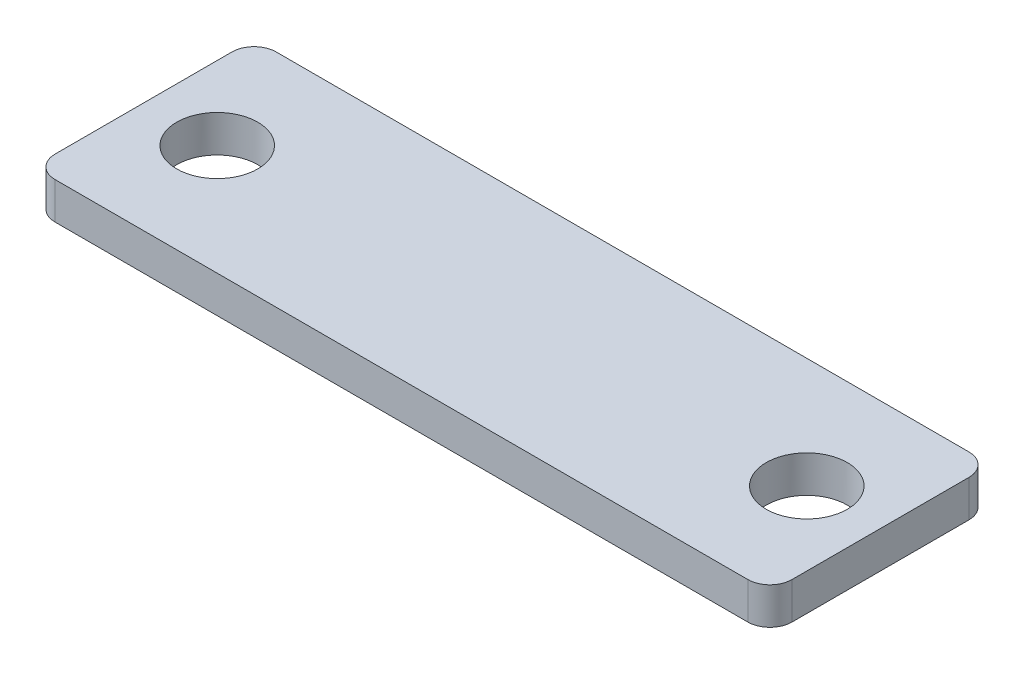
SolidWorks part; units mm, degrees
material "普通碳钢"
ref_plane "Front Plane" through (0, 0, 0) normal (0, 0, 1) x (1, 0, 0)
ref_plane "Top Plane" through (0, 0, 0) normal (0, 1, 0) x (1, 0, 0)
ref_plane "Right Plane" through (0, 0, 0) normal (1, 0, 0) x (0, 0, -1)
other "Configuration Table"
sketch "Sketch1" plane through (0, 0, 0) normal (0, 1, 0) x (1, 0, 0)
  line L1 (-50, -15) -> (50, -15)
  line L2 (-50, -15) -> (-50, 15)
  line L3 (-50, 15) -> (50, 15)
  line L4 (50, -15) -> (50, 15)
  line L5 (-50, -15) -> (50, 15) construction
  line L6 (-50, 15) -> (50, -15) construction
  point P0 (0, 0)
  dimension "D1" = 100
  dimension "D2" = 30
extrude "Boss-Extrude1" add sketch "Sketch1" along normal blind 5
fillet "Fillet1" radius 3 4 edges at (50, 2.5, 15) (50, 2.5, -15) (-50, 2.5, -15) (-50, 2.5, 15)
sketch "Sketch2" plane through (0, 5, 0) normal (0, 1, 0) x (1, 0, 0)
sketch "Sketch3" plane through (0, 5, 0) normal (0, 1, 0) x (1, 0, 0)
  line L0 (-50, 0) -> (50, 0) construction
  line L1 (-50, 12) -> (-50, -12) construction
  line L2 (50, -12) -> (50, 12) construction
  circle A0 centre (-40, 0) radius 5.5
  circle A1 centre (40, 0) radius 5.5
  dimension "D1" = 11
  dimension "D2" = 11
  dimension "D3" = 40
  dimension "D4" = 80
extrude "Cut-Extrude1" cut sketch "Sketch3" against normal blind 10
